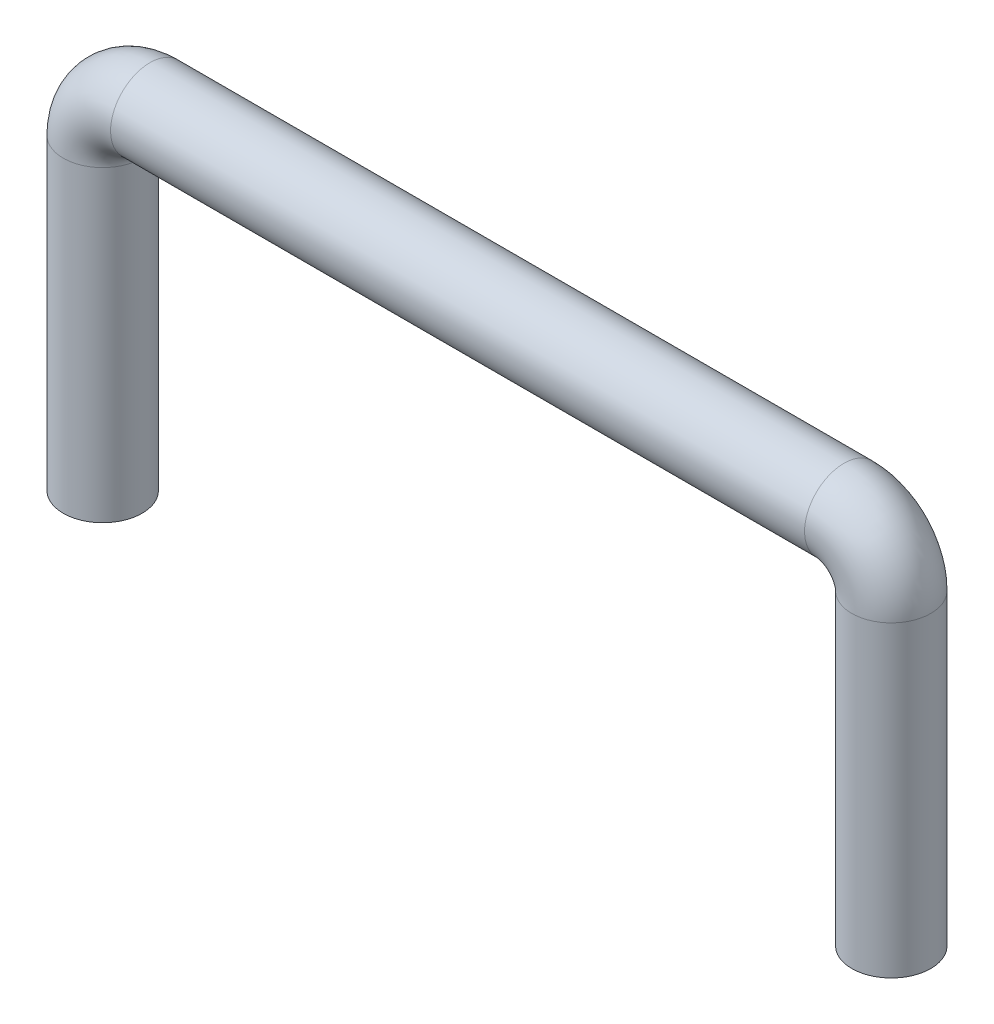
from build123d import *

# Parameters (mm, degrees)
SKETCH2_R = 5


with BuildPart() as part:
    # Sweep1: sweep along a path in Sketch1
    with BuildLine(Plane.XY) as sweep1_path:
        Line((-15.997655985, -10.44225726), (-15.997655985, 28.55774274))
        ThreePointArc((-15.997655985, 28.55774274), (-14.240296673, 32.800383427), (-9.997655985, 34.55774274))
        Line((-9.997655985, 34.55774274), (78.002344015, 34.55774274))
        ThreePointArc((78.002344015, 34.55774274), (82.244984702, 32.800383427), (84.002344015, 28.55774274))
        Line((84.002344015, 28.55774274), (84.002344015, -10.44225726))
    # Sketch2 → Sweep1 (sweep)
    with BuildSketch(Plane(origin=(-15.997655985, -10.44225726, 0), x_dir=(-1, 0, 0), z_dir=(0, 1, 0))):
        Circle(SKETCH2_R)
    sweep(path=sweep1_path.line)


solid = part.part
